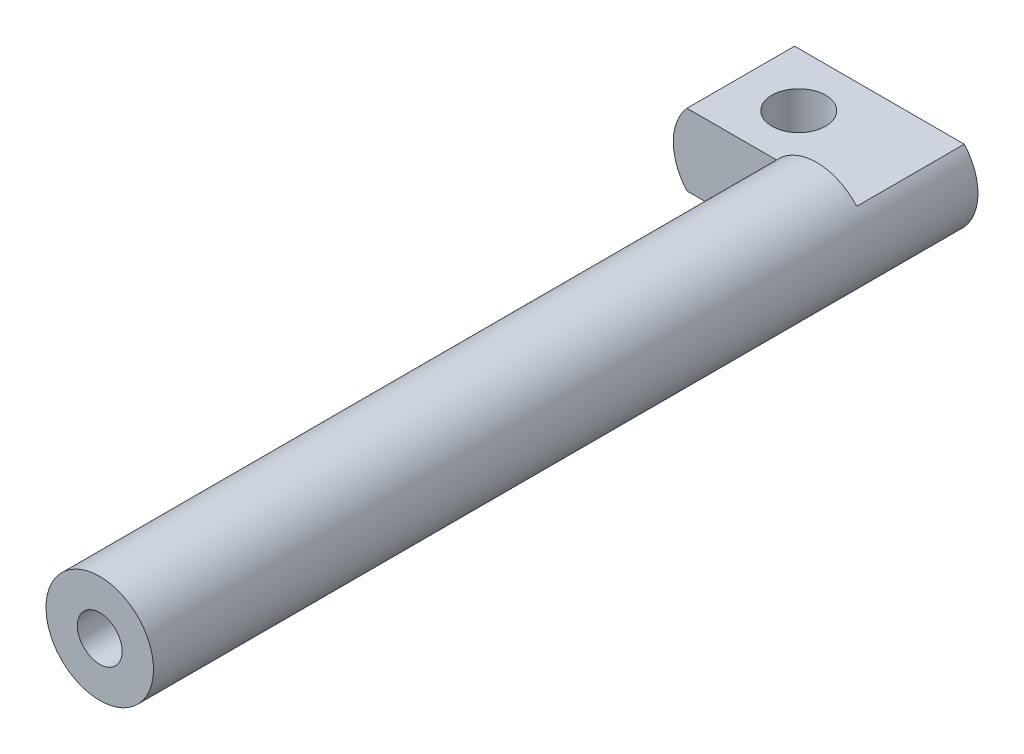
SolidWorks part; units mm, degrees
ref_plane "Front Plane" through (0, 0, 0) normal (0, 0, 1) x (1, 0, 0)
ref_plane "Top Plane" through (0, 0, 0) normal (0, 1, 0) x (1, 0, 0)
ref_plane "Right Plane" through (0, 0, 0) normal (1, 0, 0) x (0, 0, -1)
other "Configuration Table"
sketch "Sketch1" plane through (0, 0, 0) normal (0, 0, 1) x (1, 0, 0)
  circle A0 centre (0, 0) radius 3
  circle A1 centre (0, 0) radius 1.25
  dimension "D1" = 6
  dimension "D2" = 2.5
extrude "Boss-Extrude1" add sketch "Sketch1" along normal blind 40
sketch "Sketch2" plane through (0, 0, 0) normal (0, 0, -1) x (-1, 0, 0)
  line L0 (0, 0) -> (5, 0) construction
  line L1 (0, 3) -> (5, 3)
  line L2 (0, -3) -> (5, -3)
  arc A1 (0, 3) -> (0, -3) centre (0, 0) ccw
  arc A2 (5, -3) -> (5, 3) centre (5, 0) ccw
  circle A3 centre (0, 0) radius 1.25
  point P6 (2.5, 0)
  dimension "D1" = 3
  dimension "D2" = 5
extrude "Boss-Extrude2" add sketch "Sketch2" along normal blind 6
sketch "Sketch3" plane through (0, 0, -6) normal (0, 0, -1) x (-1, 0, 0)
  line L1 (-6.8132, 2) -> (9.3132, 2)
  line L2 (-6.8132, 2) -> (-6.8132, -2)
  line L3 (-6.8132, -2) -> (9.3132, -2)
  line L4 (9.3132, 2) -> (9.3132, -2)
  line L5 (-6.8132, 2) -> (9.3132, -2) construction
  line L6 (-6.8132, -2) -> (9.3132, 2) construction
  line L7 (-12.5138, 9.3362) -> (15.0138, 9.3362)
  line L8 (-12.5138, 9.3362) -> (-12.5138, -9.3362)
  line L9 (-12.5138, -9.3362) -> (15.0138, -9.3362)
  line L10 (15.0138, 9.3362) -> (15.0138, -9.3362)
  line L11 (-12.5138, 9.3362) -> (15.0138, -9.3362) construction
  line L12 (-12.5138, -9.3362) -> (15.0138, 9.3362) construction
  circle A0 centre (0, 0) radius 1.25 construction
  point P0 (1.25, 0)
  point P7 (1.25, 0)
  dimension "D1" = 4
extrude "Cut-Extrude1" cut sketch "Sketch3" against normal blind 6
sketch "Sketch4" plane through (0, -2, 0) normal (0, -1, 0) x (-1, 0, 0)
  circle A0 centre (4, 3) radius 1.5
  dimension "D1" = 3
  dimension "D2" = 4
extrude "Cut-Extrude2" cut sketch "Sketch4" against normal blind 16
